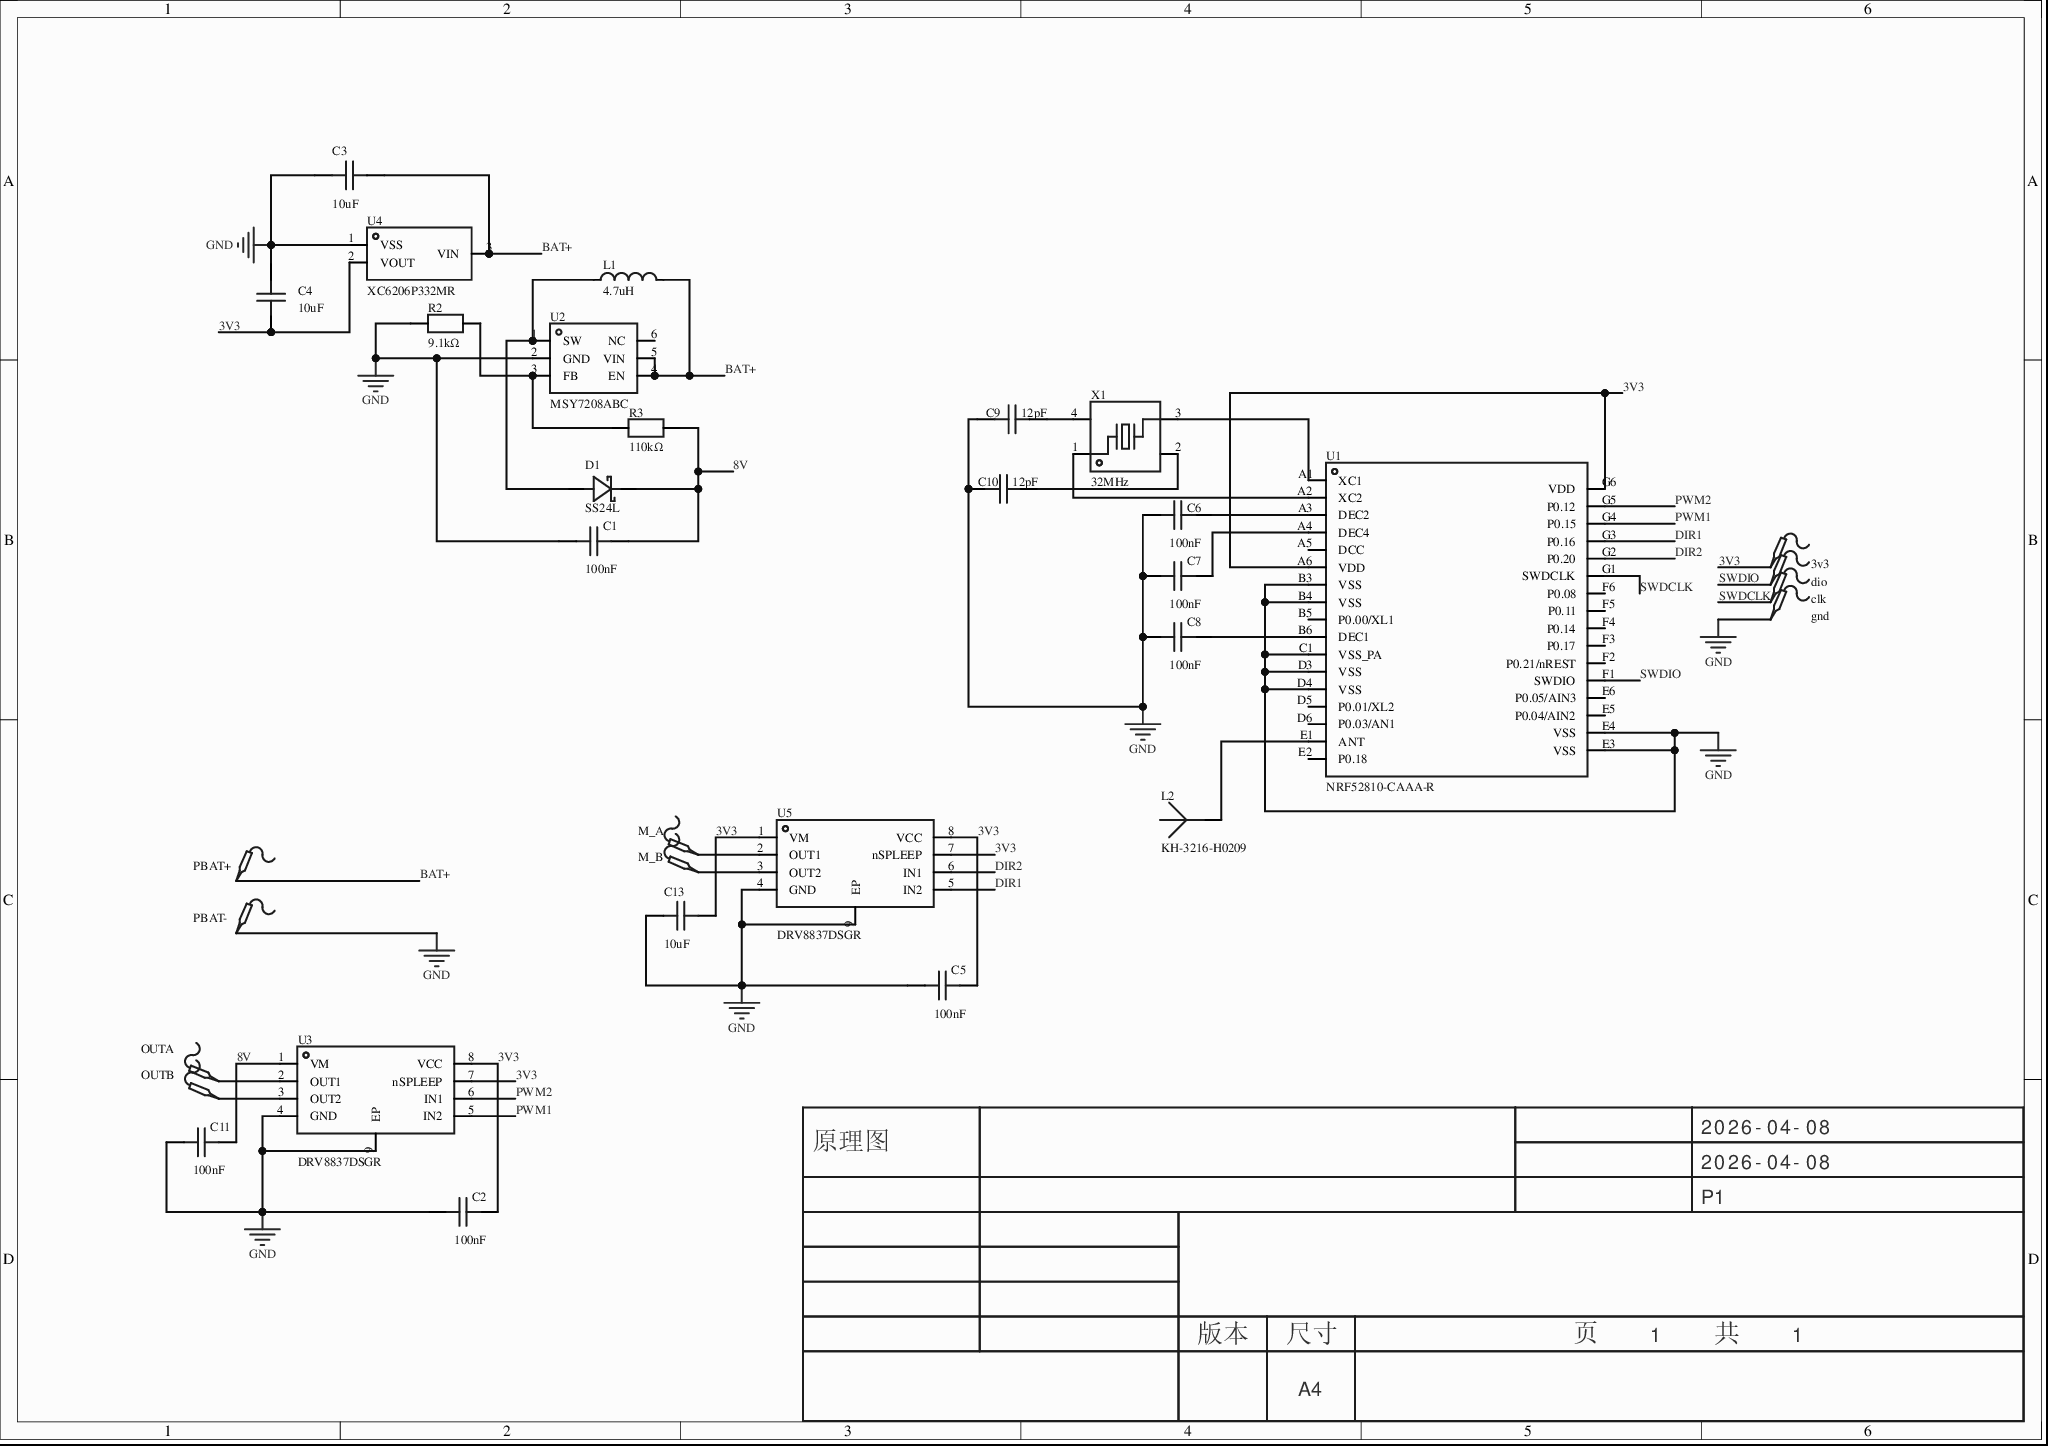
[diagram p0: MISC49870-3.schdoc]
# Altium project MISC49870-2.PrjPcb
1 sheet, 33 parts. Net scope: global (net labels, ports and power ports of the same name join across sheets).
Board file: MISC49870.pcbdoc

## Sheet MISC49870-3.schdoc
size 297 x 209 mm; Version: V1.0; @Project Name: MISC49870; @Update Date: 2026-04-08; @Create Date: 2026-04-08; @Board Name: MISC49870; @Create Time: 01:34:46; @Page Count: 1; @Page No: 1; @Schematic Name: MISC49870; @Update Time: 01:34:46; Size: A4

### Parts
3v3  (no value)  [Test-Point-0.5mm]
C1  100nF  [C0402]
C2  100nF  [C0402]
C3  10uF  [C0402]
C4  10uF  [C0402]
C5  100nF  [C0402]
C6  100nF  [C0402]
C7  100nF  [C0402]
C8  100nF  [C0402]
C9  12pF  [C0402]
C10  12pF  [C0402]
C11  100nF  [C0402]
C13  10uF  [C0402]
clk  (no value)  [Test-Point-0.5mm]
D1  SS24L  [SOD-123FL_L2.8-W1.8-LS3.7-R-RD]
dio  (no value)  [Test-Point-0.5mm]
gnd  (no value)  [Test-Point-0.5mm]
L1  4.7uH  [IND-SMD_L2.5-W2.0_VLS2520X]
L2  KH-3216-H0209  [ANT-SMD_L3.2-W1.6-KH-3216F245C04]
M_A  (no value)  [Test-Point-0.5mm]
M_B  (no value)  [Test-Point-0.5mm]
OUTA  (no value)  [Test-Point-0.5mm]
OUTB  (no value)  [Test-Point-0.5mm]
PBAT+  (no value)  [Test-Point-0.5mm]
PBAT-  (no value)  [Test-Point-0.5mm]
R2  9.1kΩ  [R0402]
R3  110kΩ  [R0402]
U1  NRF52810-CAAA-R  [WLCSP-33_L2.5-W2.5-P0.40_NRF52810-CAAA-R]
U2  MSY7208ABC  [SOT-23-6_L2.9-W1.6-P0.95-LS2.8-BR]
U3  DRV8837DSGR  [WSON-8_L2.0-W2.0-P0.50-TL-EP]
U4  XC6206P332MR  [SOT-23-3_L3.0-W1.7-P0.95-LS2.9-BR]
U5  DRV8837DSGR  [WSON-8_L2.0-W2.0-P0.50-TL-EP]
X1  32MHz  [CRYSTAL-SMD_4P-L2.0-W1.6-BL]

### Nets
GND: C1.1 C2.1 C3.1 C4.2 C5.1 C6.1 C7.1 C8.1 C9.1 C10.1 C11.1 C13.2 gnd.1 PBAT-.1 R2.1 U1.B3(VSS) U1.B4(VSS) U1.C1(VSS_PA) U1.D3(VSS) U1.D4(VSS) U1.E3(VSS) U1.E4(VSS) U2.2(GND) U3.4(GND) U3.9(EP) U4.1(VSS) U5.4(GND) U5.9(EP)
3V3: 3v3.1 C2.2 C4.1 C5.2 C13.1 U1.A6(VDD) U1.G6(VDD) U3.7(nSPLEEP) U3.8(VCC) U4.2(VOUT) U5.1(VM) U5.7(nSPLEEP) U5.8(VCC)
8V: C1.2 C11.2 D1.2(K) R3.2 U3.1(VM)
BAT+: C3.2 L1.2 PBAT+.1 U2.4(EN) U2.5(VIN) U4.3(VIN)
DIR1: U1.G3(P0.16) U5.5(IN2)
DIR2: U1.G2(P0.20) U5.6(IN1)
PWM1: U1.G4(P0.15) U3.5(IN2)
PWM2: U1.G5(P0.12) U3.6(IN1)
SWDCLK: clk.1 U1.G1(SWDCLK)
SWDIO: dio.1 U1.F1(SWDIO)
NetC6_2: C6.2 U1.A3(DEC2)
NetC7_2: C7.2 U1.A4(DEC4)
NetC8_2: C8.2 U1.B6(DEC1)
NetC9_2: C9.2 X1.4(GND)
NetC10_2: C10.2 X1.2(GND)
NetD1_1: D1.1(A) L1.1 U2.1(SW)
NetL2_1: L2.1(ANT) U1.E1(ANT)
NetM_A_1: M_A.1 U5.2(OUT1)
NetM_B_1: M_B.1 U5.3(OUT2)
NetOUTA_1: OUTA.1 U3.2(OUT1)
NetOUTB_1: OUTB.1 U3.3(OUT2)
NetR2_2: R2.2 R3.1 U2.3(FB)
NetU1_A1: U1.A1(XC1) X1.3
NetU1_A2: U1.A2(XC2) X1.1

Not connected (* = marked no-connect by the designer): L2 2; U1 A5(DCC) B5(P0.00/XL1) D5(P0.01/XL2) D6(P0.03/AN1) E2(P0.18) E5(P0.04/AIN2) E6(P0.05/AIN3) F2(P0.21/nREST) F3(P0.17) F4(P0.14) F5(P0.11) F6(P0.08); U2 6(NC)

### Notes on the sheet
- 2026-04-08
- 原理图
- P1
- 版本
- 尺寸
- A4
- 页    1    共    1

### Library data of the parts
3v3 clk dio gnd M_A M_B OUTA OUTB PBAT+ PBAT- = Test-Point: Test Point 测试点; AddInBom: yes; Symbol: Test-Point; Device: Test-Point; ConvertToPcb: yes; FootprintName: Test-Point-0.5mm
C1 C2 C6-C8 C11 = CL05B104KO5NNNC: 容值:100nF;精度:±10%;额定电压:16V;温度系数:X7R;; Manufacturer: SAMSUNG(三星); AddInBom: yes; ModelId: 36a51122f27c49738f86b3bfa98863e00819f05c4eef4c71ace90d822a990e87; ModelName: C0402_L1.0-W0.5-H0.5; ModelTransform: 39.37,19.685,0,0,0,0,0,0,0; Tolerance: ±10%; Voltage Rating: 16V; Temperature Coefficient: X7R; Symbol: CL05B104KO5NNNC; Device: CL05B104KO5NNNC; LCSC Part Name: 100nF ±10% 16V; SupplierPart: C1525; ManufacturerPart: CL05B104KO5NNNC; Supplier Footprint: 0402; JLCPCB Part Class: Basic Part; Datasheet: https://item.szlcsc.com/datasheet/CL05B104KO5NNNC/1877.html; Supplier: LCSC; ConvertToPcb: yes; FootprintName: C0402; Value: 100nF
C3 C4 = CGA0402X5R106M100GT: 容值:10uF;精度:±20%;额定电压:10V;温度系数:X5R;; Manufacturer: HRE(芯声); AddInBom: yes; ModelId: 36a51122f27c49738f86b3bfa98863e00819f05c4eef4c71ace90d822a990e87; ModelName: C0402_L1.0-W0.5-H0.5; ModelTransform: 39.37,19.685,0,0,0,0,0,0,0; Tolerance: ±20%; Voltage Rating: 10V; Temperature Coefficient: X5R; Symbol: CGA0402X5R106M100GT; Device: CGA0402X5R106M100GT; LCSC Part Name: 10uF ±20% 10V; SupplierPart: C6119763; ManufacturerPart: CGA0402X5R106M100GT; Supplier Footprint: 0402; JLCPCB Part Class: Extended Part; Datasheet: https://item.szlcsc.com/datasheet/CGA0402X5R106M100GT/7062469.html; Supplier: LCSC; ConvertToPcb: yes; FootprintName: C0402; Value: 10uF
C5 = CL05B104KO5NNNC: 容值:100nF;精度:±10%;额定电压:16V;温度系数:X7R;; Manufacturer: SAMSUNG(三星); 3D Model: 36a51122f27c49738f86b3bfa98863e00819f05c4eef4c71ace90d822a990e87; 3D Model Transform: 39.37,19.685,0,0,0,0,0,0,0; Tolerance: ±10%; Voltage Rating: 16V; Temperature Coefficient: X7R; AddInBom: yes; ModelName: C0402_L1.0-W0.5-H0.5; Symbol: CL05B104KO5NNNC; Device: CL05B104KO5NNNC; LCSC Part Name: 100nF ±10% 16V; Supplier Part: C1525; Manufacturer Part: CL05B104KO5NNNC; Supplier Footprint: 0402; JLCPCB Part Class: Basic Part; Datasheet: https://item.szlcsc.com/datasheet/CL05B104KO5NNNC/1877.html; Supplier: LCSC; Value: 100nF; ConvertToPcb: yes; FootprintName: C0402
C9 C10 = CGA0402C0G120J500GT: 容值:12pF;精度:±5%;额定电压:50V;温度系数:C0G;; Manufacturer: HRE(芯声); AddInBom: yes; ModelId: 36a51122f27c49738f86b3bfa98863e00819f05c4eef4c71ace90d822a990e87; ModelName: C0402_L1.0-W0.5-H0.5; ModelTransform: 39.37,19.685,0,0,0,0,0,0,0; Tolerance: ±5%; Voltage Rating: 50V; Temperature Coefficient: C0G; Symbol: CGA0402C0G120J500GT; Device: CGA0402C0G120J500GT; LCSC Part Name: 12pF ±5% 50V; SupplierPart: C45359894; ManufacturerPart: CGA0402C0G120J500GT; Supplier Footprint: 0402; JLCPCB Part Class: Extended Part; Datasheet: https://item.szlcsc.com/datasheet/CGA0402C0G120J500GT/47452244.html; Supplier: LCSC; ConvertToPcb: yes; FootprintName: C0402; Value: 12pF
C13 = CGA0402X5R106M100GT: 容值:10uF;精度:±20%;额定电压:10V;温度系数:X5R;; Manufacturer: HRE(芯声); 3D Model: 36a51122f27c49738f86b3bfa98863e00819f05c4eef4c71ace90d822a990e87; 3D Model Transform: 39.37,19.685,0,0,0,0,0,0,0; Tolerance: ±20%; Voltage Rating: 10V; Temperature Coefficient: X5R; AddInBom: yes; ModelName: C0402_L1.0-W0.5-H0.5; Symbol: CGA0402X5R106M100GT; Device: CGA0402X5R106M100GT; LCSC Part Name: 10uF ±20% 10V; Supplier Part: C6119763; Manufacturer Part: CGA0402X5R106M100GT; Supplier Footprint: 0402; JLCPCB Part Class: Extended Part; Datasheet: https://item.szlcsc.com/datasheet/CGA0402X5R106M100GT/7062469.html; Supplier: LCSC; Value: 10uF; ConvertToPcb: yes; FootprintName: C0402
D1 = SS24L_C2827931: 二极管配置:独立式;正向压降(Vf):500mV@2A;直流反向耐压(Vr):40V;整流电流:2A;; Manufacturer: Hottech(合科泰); AddInBom: yes; ModelId: 8393683a03e6444f97e03ed1558f3a520819f05c4eef4c71ace90d822a990e87; ModelTransform: 143.701,70.3249,0,0,0,0,0,0,0; Diode Configuration: 独立式; Voltage - DC Reverse(Vr): 40V; Current - Rectified: 2A; Reverse Leakage Current (Ir): 500uA@40V; Non-Repetitive Peak Forward Surge Current: 50A; Symbol: SS24L; Device: SS24L_C2827931; LCSC Part Name: 电压:40V 电流:2A; SupplierPart: C2827931; ManufacturerPart: SS24L; Supplier Footprint: SOD-123FL; JLCPCB Part Class: Extended Part; Datasheet: https://item.szlcsc.com/datasheet/SS24L/2974958.html; Supplier: LCSC; ConvertToPcb: yes; FootprintName: SOD-123FL_L2.8-W1.8-LS3.7-R-RD; ModelName: SOD-123FL_L2.8-W1.8-LS3.7-R-RD; Voltage - Forward(Vf@If): 500mV@2A
L1 = VLS252012CX-4R7M: 电感值:4.7uH;精度:±20%;饱和电流(Isat):1.1A;; Manufacturer: TDK; AddInBom: yes; ModelId: 81d5beb8ff1341c89c4ff52d6c0040bf0819f05c4eef4c71ace90d822a990e87; ModelName: IND-SMD_L2.5-W2.0-H1.2_VLS2520X; ModelTransform: 98.425,79.61023,0,0,0,0,0,0,0; Tolerance: ±20%; Saturation Current (Isat): 1.1A; DC Resistance (DCR): 210mΩ; Symbol: VLS252012CX-4R7M; Device: VLS252012CX-4R7M; LCSC Part Name: 4.7uH ±20% 1.1A; SupplierPart: C6323073; ManufacturerPart: VLS252012CX-4R7M; Supplier Footprint: 2520; JLCPCB Part Class: Extended Part; Datasheet: https://atta.szlcsc.com/upload/public/pdf/source/20241101/1B0DCD755C10F25FE430CD0DF989EC97.pdf; Supplier: LCSC; ConvertToPcb: yes; FootprintName: IND-SMD_L2.5-W2.0_VLS2520X; Value: 4.7uH
L2 = KH-3216-H0209: 天线类型:贴片天线;中心频率:2.45GHz;带宽:120MHz;增益:1.71dBi;功率:4W;; Manufacturer: kinghelm(金航标); AddInBom: yes; ModelId: b0a58d898f8d48158173012e6d49bb4f0819f05c4eef4c71ace90d822a990e87; ModelTransform: 127.9525,65.354,0,0,0,0,0,0,0; Antenna Type: 贴片天线; Bandwidth: 120MHz; Impedance: 50Ω; Power: 4W; Symbol: KH-3216-H0209; Device: KH-3216-H0209; LCSC Part Name: 3216 Chip antenna，2.4~2.5GHz，适用于蓝牙/WLAN应用; SupplierPart: C2925417; ManufacturerPart: KH-3216-H0209; Supplier Footprint: 1206; JLCPCB Part Class: Extended Part; Datasheet: https://item.szlcsc.com/datasheet/KH-3216-H0209/3244679.html; Supplier: LCSC; ConvertToPcb: yes; FootprintName: ANT-SMD_L3.2-W1.6-KH-3216F245C04; ModelName: ANT-SMD_L3.2-W1.6-KH-3216F245C04; Frequency(Center/Band): 2.45GHz; Peak Gain: 1.71dBi; Operating Temperature: -40℃~+110℃; Length: 3.23mm; Width: 1.66mm; Height: 0.45mm
R2 = FRC0402F9101TS: 电阻类型:厚膜电阻;阻值:9.1kΩ;精度:±1%;功率:62.5mW;工作电压:50V;温度系数:±100ppm/℃;; Manufacturer: FOJAN(富捷); AddInBom: yes; ModelId: 98c88bc2b9094f218f3a3e30a70127380819f05c4eef4c71ace90d822a990e87; ModelName: R0402_L1.0-W0.5-H0.4; ModelTransform: 39.37,19.685,0,0,0,0,0,0,0; Tolerance: ±1%; Power(Watts): 62.5mW; Voltage-Supply(Max): 50V; Symbol: FRC0402F9101TS; Device: FRC0402F9101TS; LCSC Part Name: 9.1kΩ ±1% 62.5mW 厚膜电阻; SupplierPart: C2909390; ManufacturerPart: FRC0402F9101TS; Supplier Footprint: 0402; JLCPCB Part Class: Extended Part; Datasheet: https://item.szlcsc.com/datasheet/FRC0402F9101TS/3186325.html; Supplier: LCSC; ConvertToPcb: yes; FootprintName: R0402; Type: 厚膜电阻; Value: 9.1kΩ; Temperature Coefficient: ±100ppm/℃; Operating Temperature: -55℃~+155℃
R3 = FRC0402F1103TS: 电阻类型:厚膜电阻;阻值:110kΩ;精度:±1%;功率:62.5mW;工作电压:50V;温度系数:±100ppm/℃;; Manufacturer: FOJAN(富捷); AddInBom: yes; ModelId: 98c88bc2b9094f218f3a3e30a70127380819f05c4eef4c71ace90d822a990e87; ModelName: R0402_L1.0-W0.5-H0.4; ModelTransform: 39.37,19.685,0,0,0,0,0,0,0; Tolerance: ±1%; Power(Watts): 62.5mW; Voltage-Supply(Max): 50V; Symbol: FRC0402F1103TS; Device: FRC0402F1103TS; LCSC Part Name: 110kΩ ±1% 62.5mW 厚膜电阻; SupplierPart: C2909311; ManufacturerPart: FRC0402F1103TS; Supplier Footprint: 0402; JLCPCB Part Class: Extended Part; Supplier: LCSC; ConvertToPcb: yes; FootprintName: R0402; Type: 厚膜电阻; Value: 110kΩ; Temperature Coefficient: ±100ppm/℃; Operating Temperature: -55℃~+155℃
U1 = NRF52810-CAAA-R: 频率范围:-;接口类型:ADC；PWM；UART；PDM；SPI;应用领域:蓝牙;数据速率:2Mbps;灵敏度:-96dBm;典型应用频率:2.4GHz;; Manufacturer: NORDIC; AddInBom: yes; Voltage - Supply: 1.7V~3.6V; Output Power: 4dBm; Data Rate: 2Mbps; Current Of Transmitting: 4.6mA; Sensitivity: -96dBm; Typical Application Frequency: 2.4GHz; Symbol: NRF52810-CAAA-R; Device: NRF52810-CAAA-R; LCSC Part Name: 2.4 GHz收发器，支持多协议; SupplierPart: C3606661; ManufacturerPart: NRF52810-CAAA-R; Supplier Footprint: WLCSP-33(2.5x2.5); JLCPCB Part Class: Extended Part; Datasheet: https://item.szlcsc.com/datasheet/NRF52810-CAAA-R/4173388.html; Supplier: LCSC; ConvertToPcb: yes; FootprintName: WLCSP-33_L2.5-W2.5-P0.40_NRF52810-CAAA-R; Frequency Range: -; Interface: ADC；PWM；UART；PDM；SPI; Applications: 蓝牙; Receive Current: 4.6mA; Operating Temperature: -40℃~+85℃; Type: 收发器
U2 = MSY7208ABC: 功能类型:升压型;工作电压:2.5V~24V;输出类型:可调;; Manufacturer: MSKSEMI(美森科); AddInBom: yes; ModelId: 18da8f6c14a34920b3e136b5c401a1190819f05c4eef4c71ace90d822a990e87; ModelName: SOT-23-6_L2.9-W1.6-H1.5-LS2.8-P0.95; ModelTransform: 110.73671,114.173,0,180,0,0,0.001,-0.003,0; Function: 升压型; Frequency - Switching: 1.2MHz; Number of Outputs: 1; Topology: 升压式; Quiescent Current: 70uA; Switch tube (built-in/external): 内置; Output Type: 可调; Symbol: MSY7208ABC; Device: MSY7208ABC; LCSC Part Name: MSY7208ABC; SupplierPart: C49375257; ManufacturerPart: MSY7208ABC; Supplier Footprint: SOT-23-6; JLCPCB Part Class: Extended Part; Datasheet: https://item.szlcsc.com/datasheet/MSY7208ABC/51886969.html; Supplier: LCSC; ConvertToPcb: yes; FootprintName: SOT-23-6_L2.9-W1.6-P0.95-LS2.8-BR; Voltage - Supply: 2.5V~24V
U3 = DRV8837DSGR: DRV8837 12V、1.8A H 桥电机驱动器; Manufacturer: TI(德州仪器); AddInBom: yes; ModelId: 2d2152581c994cd984cd640674c19dc70819f05c4eef4c71ace90d822a990e87; ModelName: WSON-8_L2.0-W2.0-H0.8-P0.50; ModelTransform: 79.527,78.74,0,0,0,0,0,0,0; Peak Current: 1.9A; Voltage - Supply: 1.8V~7V; RDS(on): 280mΩ; Quiescent Current(Iq): 120nA; Symbol: DRV8837DSGR; Device: DRV8837DSGR; LCSC Part Name: 1.8A 有刷直流电机驱动芯片 7V; SupplierPart: C39159; ManufacturerPart: DRV8837DSGR; Supplier Footprint: WSON-8-EP(2x2); JLCPCB Part Class: Extended Part; Datasheet: https://www.ti.com/cn/lit/gpn/drv8837; Supplier: LCSC; ConvertToPcb: yes; FootprintName: WSON-8_L2.0-W2.0-P0.50-TL-EP; Technology: 是; Number of H-bridges: -; Output Current: -; Interface: -; Operating Temperature: -40℃~+85℃
U4 = XC6206P332MR_C347376: 输出类型:固定;工作电压:8V;输出电压:3.3V;输出电流:250mA;电源纹波抑制比(PSRR):40dB@(1kHz);输出极性:正极;; Manufacturer: UMW(友台半导体); AddInBom: yes; ModelId: 89cb27a44ab2466697082bb9fd73a7d00819f05c4eef4c71ace90d822a990e87; ModelName: SOT-23-3L_L2.9-W1.6-H1.1-LS2.8-P0.95; ModelTransform: 114.173,110.236,0,90,0,0,0,0,0; Output Type: 固定; Voltage - Supply: 8V; Output Voltage: 3.3V; Output Current: 250mA; Voltage Dropout: 240mV@(50mA); standby current: 7uA; Output Configuration: 正极; Number of Outputs: 1; Symbol: XC6206P332MR_C347376; Device: XC6206P332MR_C347376; LCSC Part Name: 高纹波抑制率、低功耗、低压差 CMOS 降压型电压稳压器; SupplierPart: C347376; ManufacturerPart: XC6206P332MR; Supplier Footprint: SOT-23; JLCPCB Part Class: Extended Part; Datasheet: https://item.szlcsc.com/datasheet/XC6206P332MR/324036.html; Supplier: LCSC; ConvertToPcb: yes; FootprintName: SOT-23-3_L3.0-W1.7-P0.95-LS2.9-BR; Power Supply Rejection Ratio (PSRR): 40dB@(1kHz); Noise: -; Features: 过流保护；短路保护; Operating Temperature: -25℃~+80℃@(Ta)
U5 = DRV8837DSGR: DRV8837 12V、1.8A H 桥电机驱动器; Manufacturer: TI(德州仪器); 3D Model: 2d2152581c994cd984cd640674c19dc70819f05c4eef4c71ace90d822a990e87; 3D Model Transform: 79.527,78.74,0,0,0,0,0,0,0; Peak Current: 1.9A; Voltage - Supply: 1.8V~7V; RDS(on): 280mΩ; Quiescent Current(Iq): 120nA; AddInBom: yes; ModelName: WSON-8_L2.0-W2.0-H0.8-P0.50; Symbol: DRV8837DSGR; Device: DRV8837DSGR; LCSC Part Name: 1.8A 有刷直流电机驱动芯片 7V; Supplier Part: C39159; Manufacturer Part: DRV8837DSGR; Supplier Footprint: WSON-8-EP(2x2); JLCPCB Part Class: Extended Part; Datasheet: https://www.ti.com/cn/lit/gpn/drv8837; Supplier: LCSC; Technology: 是; Number of H-bridges: -; Output Current: -; Interface: -; Operating Temperature: -40℃~+85℃; ConvertToPcb: yes; FootprintName: WSON-8_L2.0-W2.0-P0.50-TL-EP
X1 = XL7EL89CKI-111YLC-32M: 晶振类型:贴片晶振;频率:32MHz;常温频差:±10ppm;负载电容:8pF;频率稳定度:±20ppm;; Manufacturer: YXC(扬兴晶振); AddInBom: yes; ModelId: 5d2c7f6d96ec4dd1b062bb930f1f4d300819f05c4eef4c71ace90d822a990e87; ModelTransform: 80.709,64.961,0,0,0,0,0,0,0; Normal temperature Frequency Tolerance: ±10ppm; Load Capacitance: 8pF; Frequency Stability: ±20ppm; Symbol: XL7EL89CKI-111YLC-32M; Device: XL7EL89CKI-111YLC-32M; LCSC Part Name: YSX211SL 32MHZ 4P 2016 8PF ±10PPM -40~85℃ (±20PPM); SupplierPart: C2965582; ManufacturerPart: XL7EL89CKI-111YLC-32M; Supplier Footprint: SMD2016-4P; JLCPCB Part Class: Extended Part; Datasheet: https://item.szlcsc.com/datasheet/XL7EL89CKI-111YLC-32M/3357718.html; Supplier: LCSC; ConvertToPcb: yes; FootprintName: CRYSTAL-SMD_4P-L2.0-W1.6-BL; ModelName: CRYSTAL-SMD_4P-L2.0-W1.6-BL; Type: 贴片晶振; Value: 32MHz; Equivalent Series Resistance(ESR): -; Operating Temperature: -40℃~+85℃